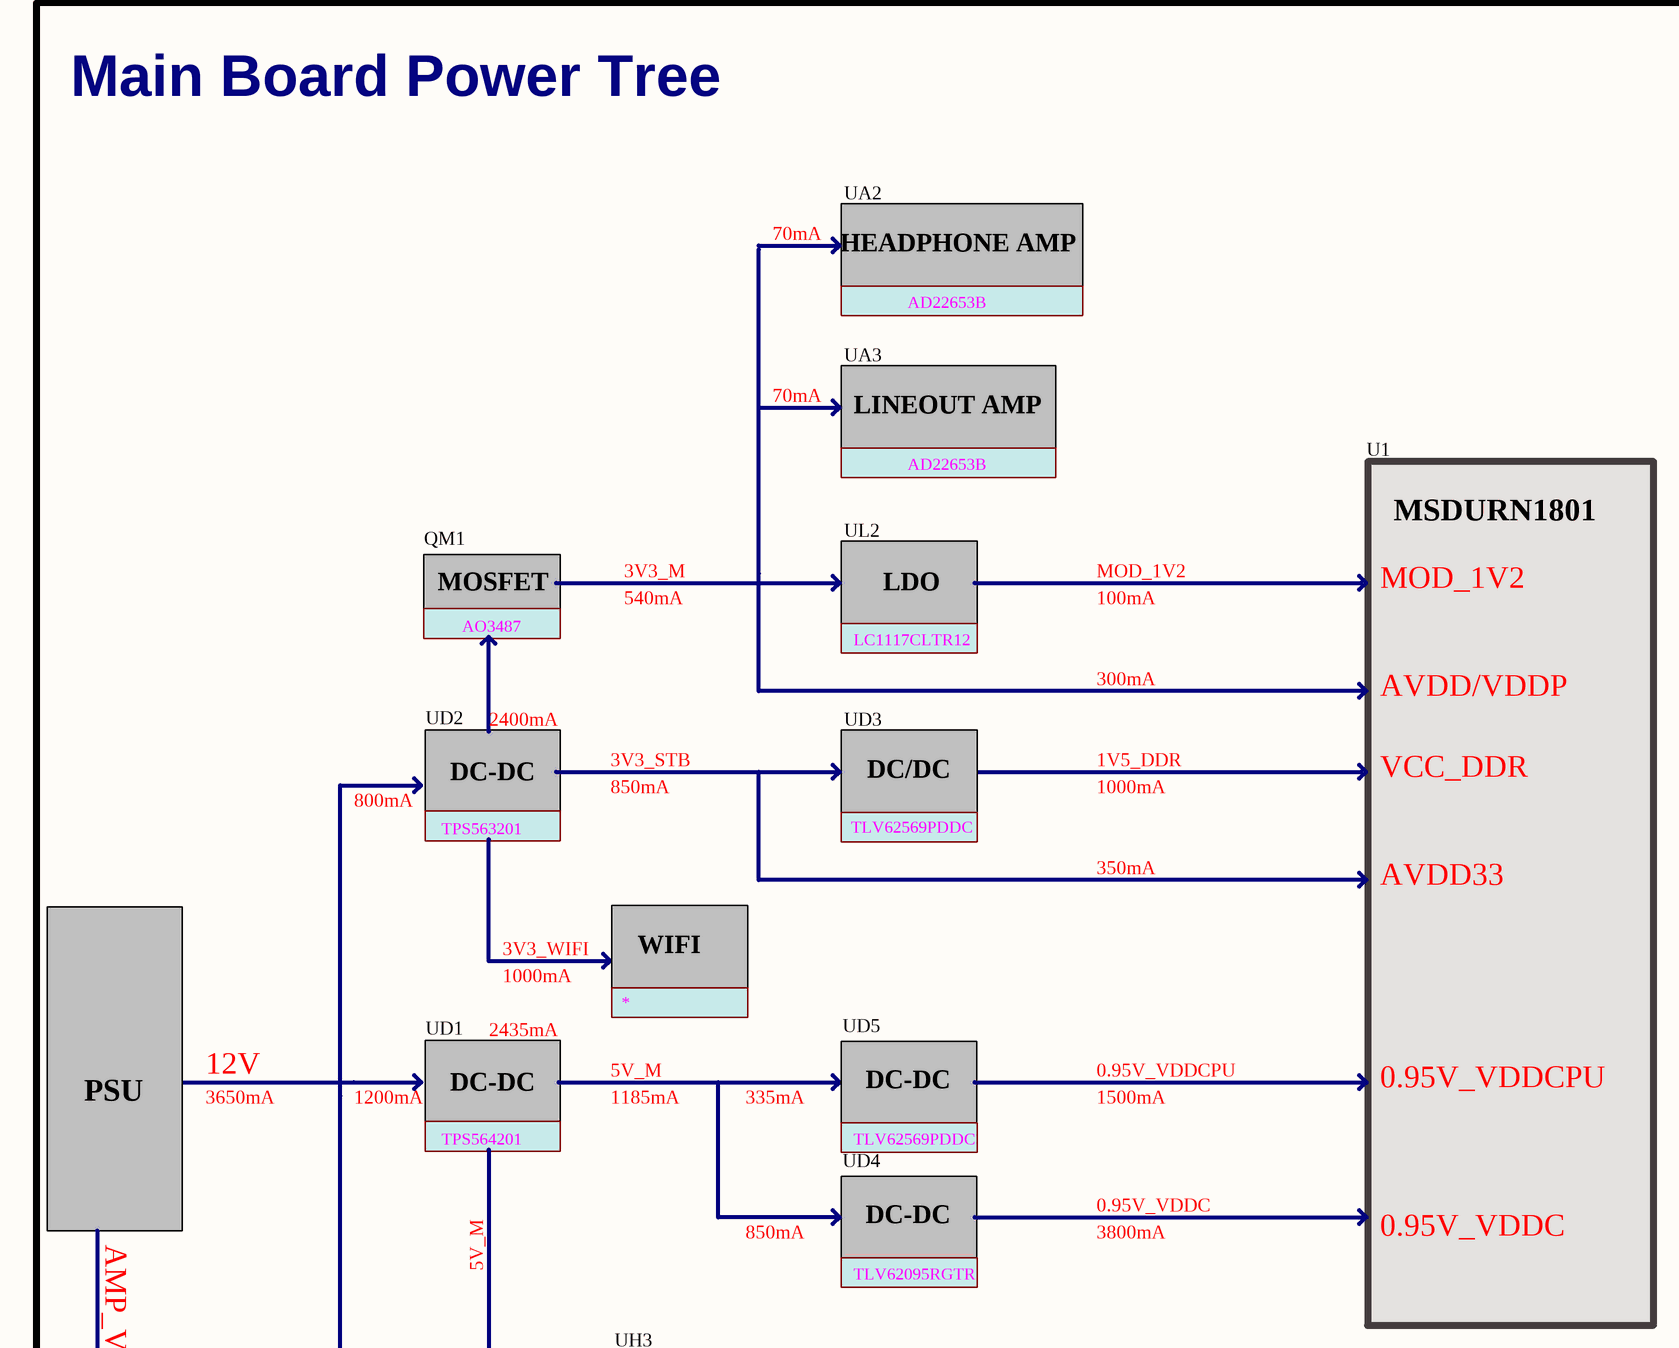
[diagram p0: MISC86290-5.SchDoc, top left]
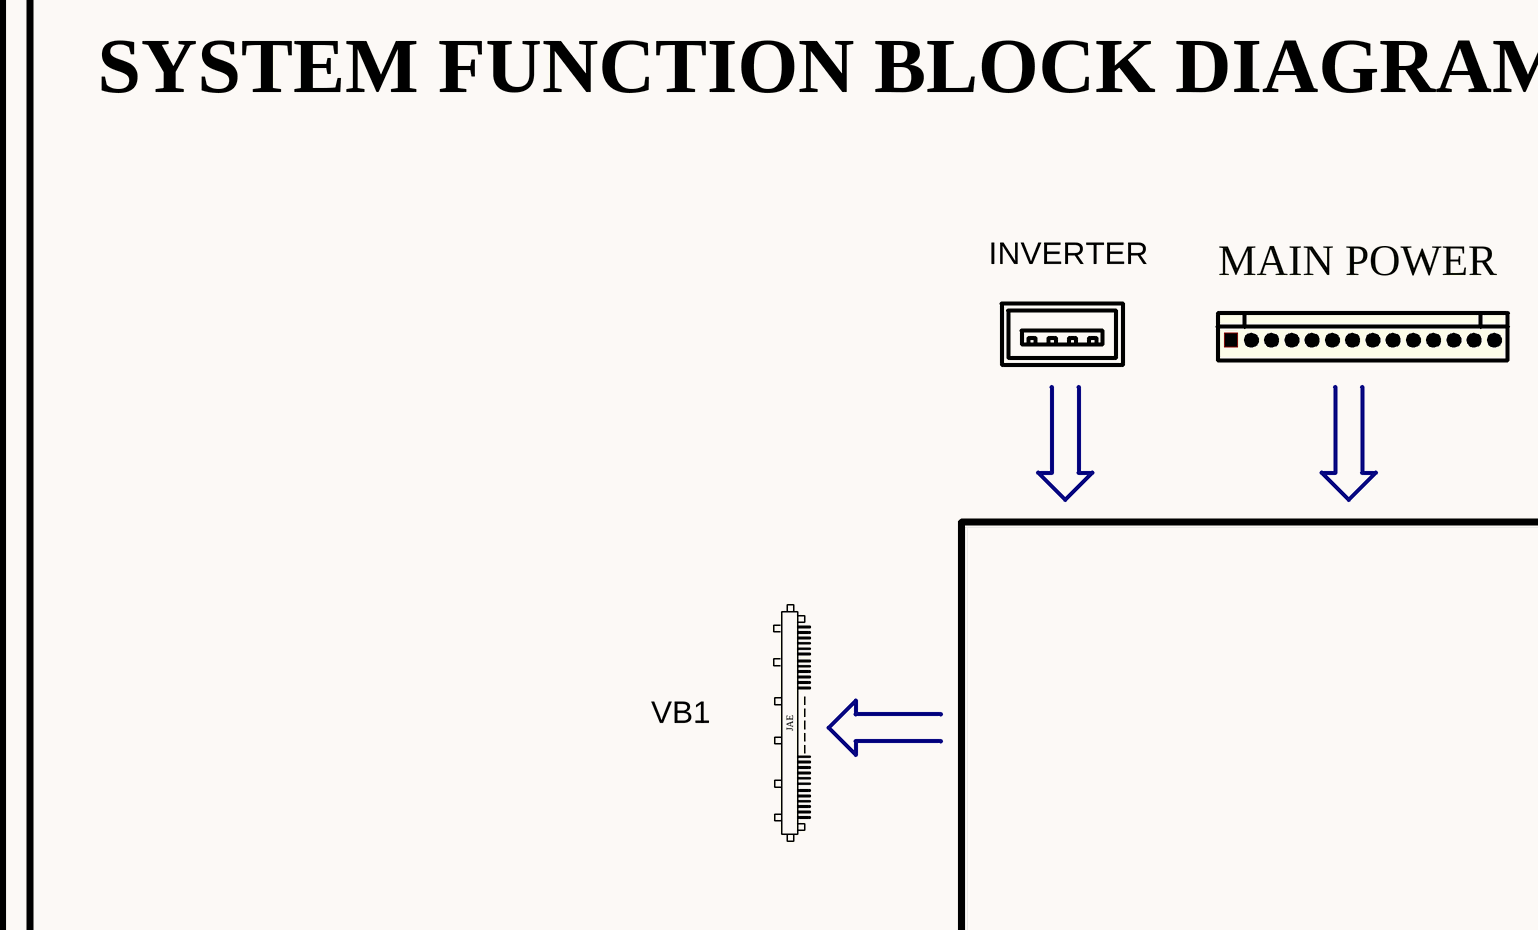
[diagram p1: MISC86290-5.SchDoc, top middle]
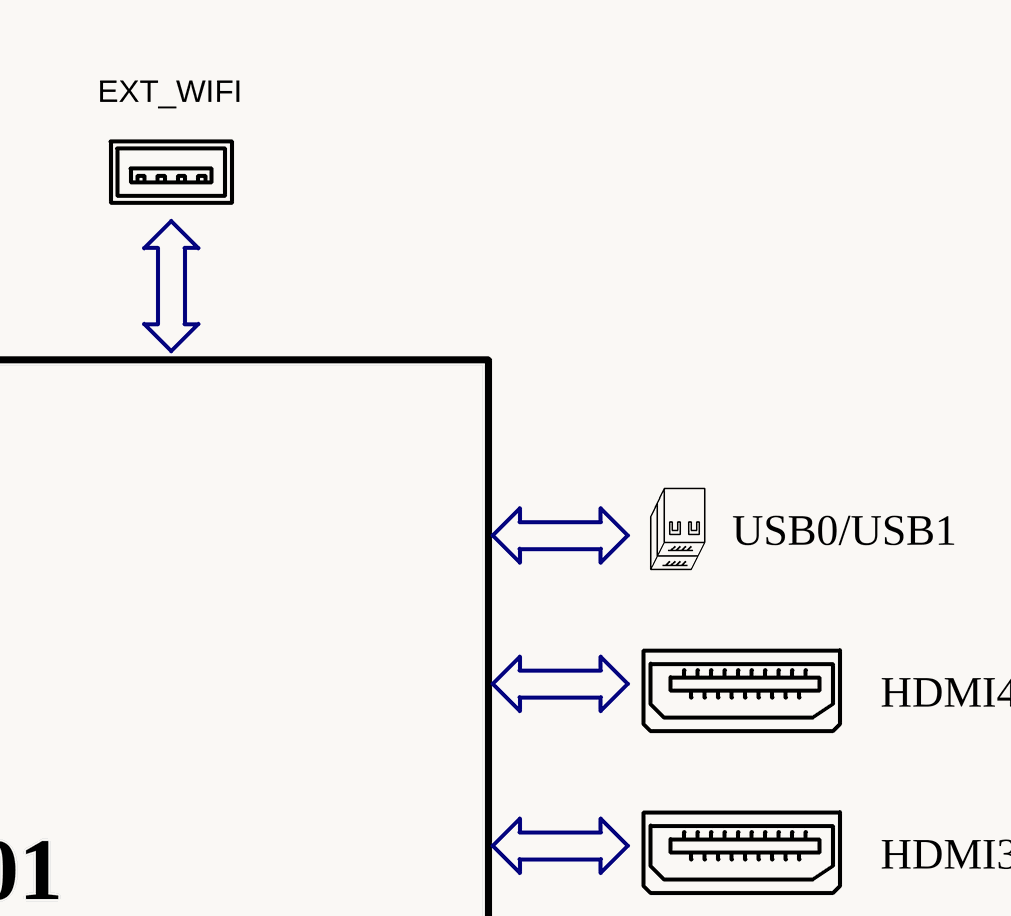
[diagram p2: MISC86290-5.SchDoc, top right]
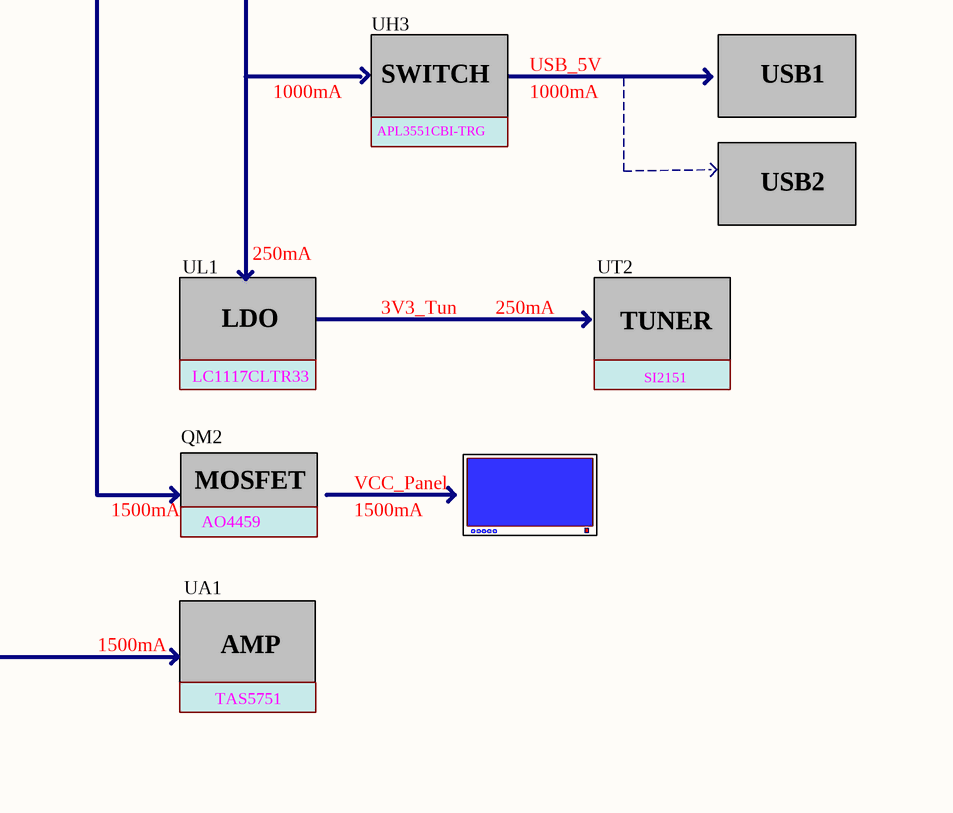
[diagram p3: MISC86290-5.SchDoc, bottom left]
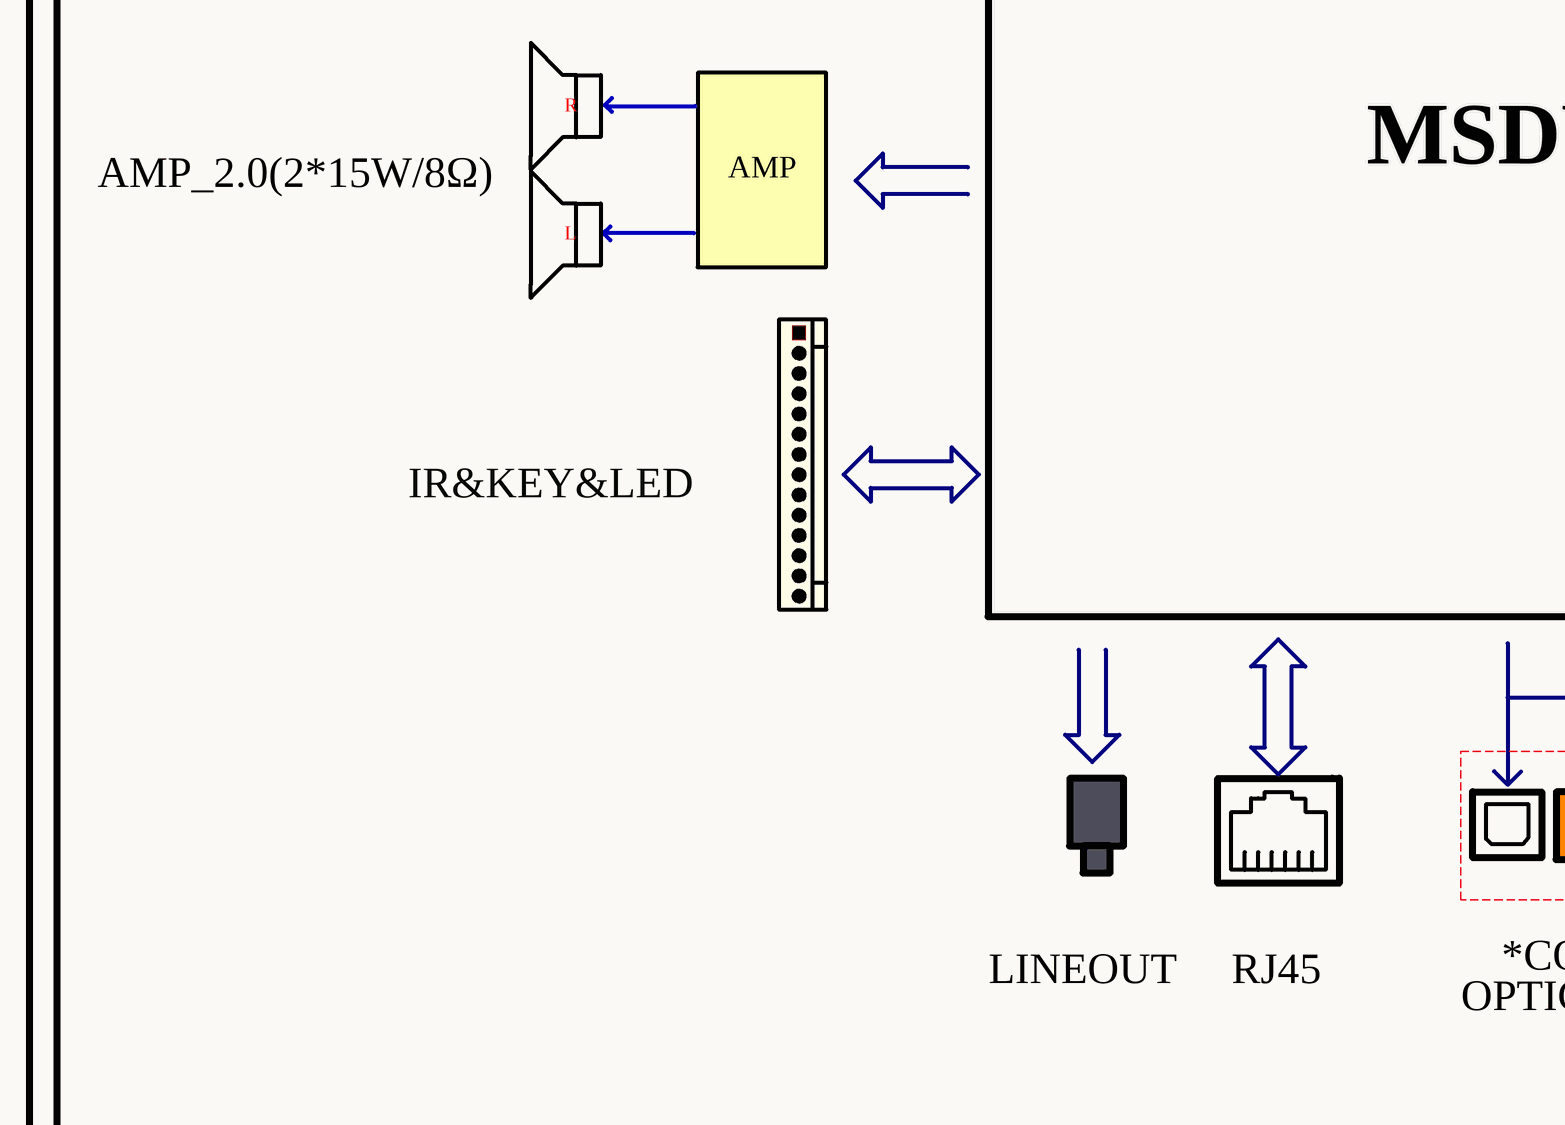
[diagram p4: MISC86290-5.SchDoc, bottom middle]
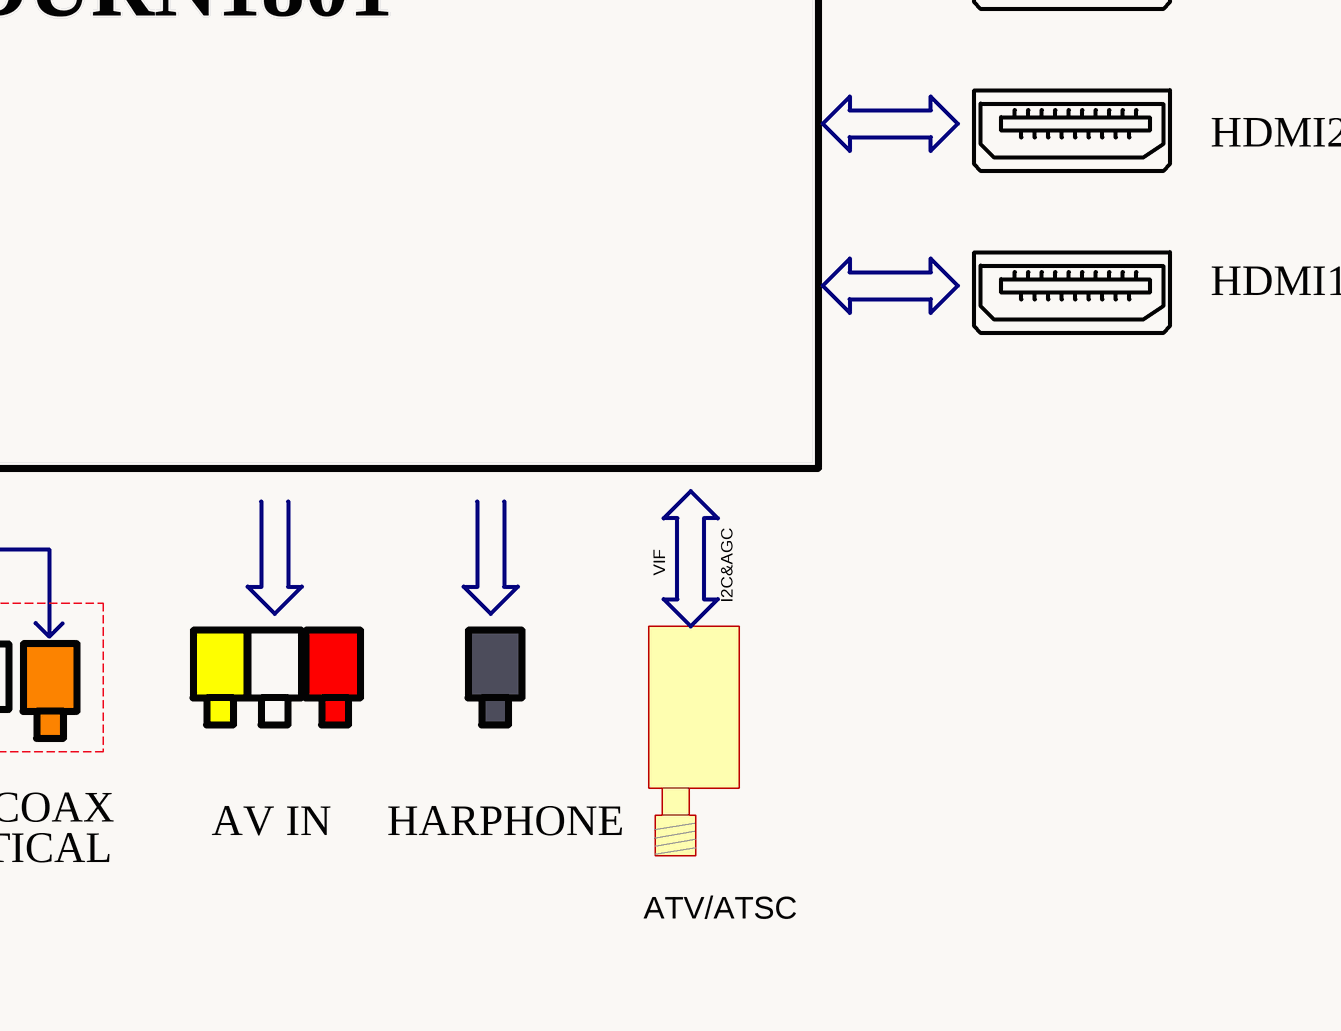
[diagram p5: MISC86290-5.SchDoc, bottom right]
# Altium project MISC86290.PrjPcb (part 2 of 13)

## Sheet MISC86290-5.SchDoc
size 889 x 426 mm